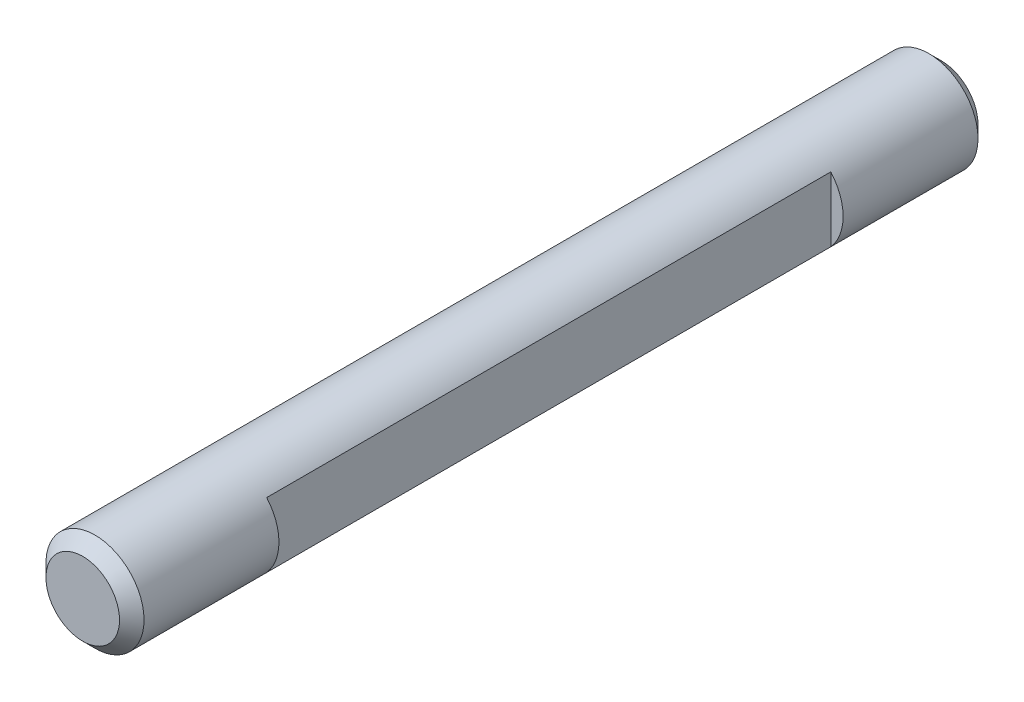
SolidWorks part; units mm, degrees
material "硬光轴"
ref_plane "Front Plane" through (0, 0, 0) normal (0, 0, 1) x (1, 0, 0)
ref_plane "Top Plane" through (0, 0, 0) normal (0, 1, 0) x (1, 0, 0)
ref_plane "Right Plane" through (0, 0, 0) normal (1, 0, 0) x (0, 0, -1)
sketch "Sketch1" plane through (0, 0, 0) normal (0, 0, 1) x (1, 0, 0)
  circle A0 centre (0, 0) radius 2
  dimension "D1" = 4
extrude "Boss-Extrude1" add sketch "Sketch1" along normal mid plane 35
chamfer "Chamfer1" distance 0.5 angle 45 2 edges at (2, 0, -17.5) (2, 0, 17.5)
sketch "Sketch2" plane through (0, 0, 0) normal (0, 1, 0) x (1, 0, 0)
  line L0 (2, -17) -> (2, 17) construction
  line L1 (2.5, -11.5) -> (1.5, -11.5)
  line L2 (2.5, -11.5) -> (2.5, 11.5)
  line L3 (2.5, 11.5) -> (1.5, 11.5)
  line L4 (1.5, -11.5) -> (1.5, 11.5)
  line L5 (2.5, -11.5) -> (1.5, 11.5) construction
  line L6 (2.5, 11.5) -> (1.5, -11.5) construction
  point P0 (2, 0)
  dimension "D1" = 23
  dimension "D2" = 1
extrude "Cut-Extrude1" cut sketch "Sketch2" against normal mid plane 10
